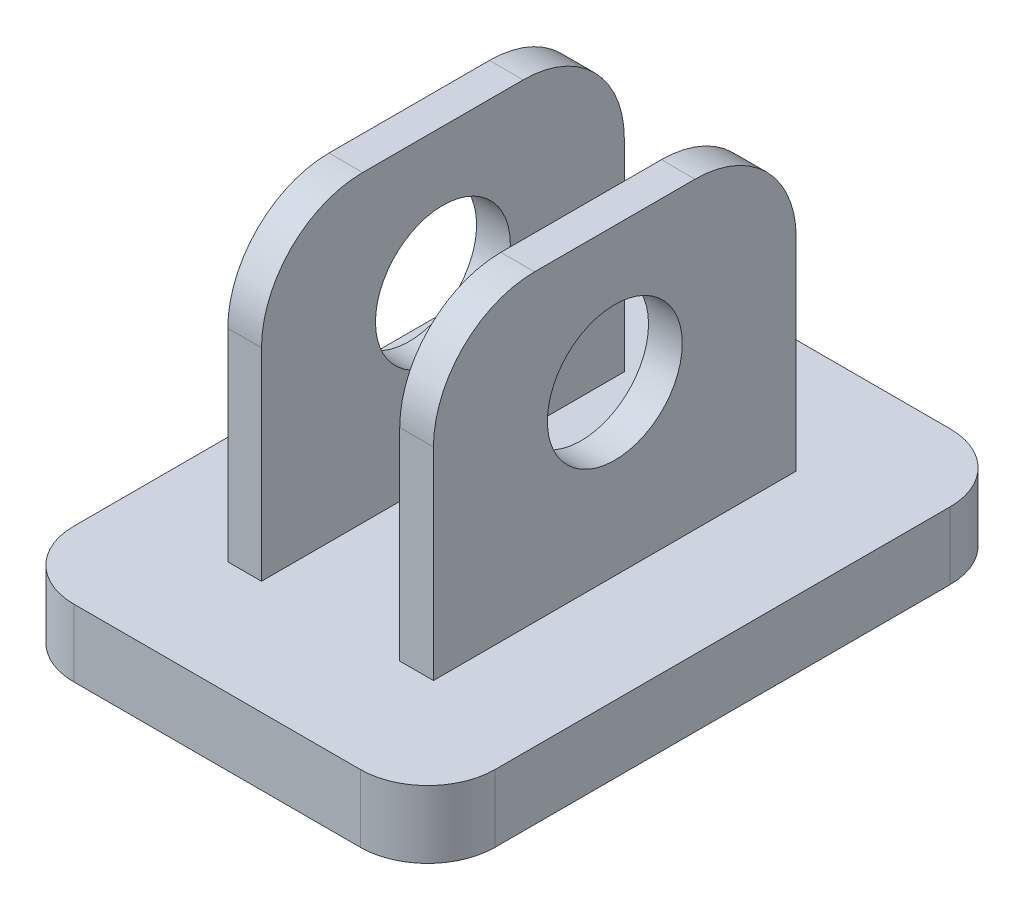
from build123d import *

# Parameters (mm, degrees)
BOSS_EXTRU_1_DEPTH = 4
SKETCH2_W          = 2
SKETCH2_H          = 21.522663516
BOSS_EXTRU_2_DEPTH = 18
FILLET1_R          = 6
SKETCH3_R          = 4
CUT_EXTRUDE1_DEPTH = 34.707714251


with BuildPart() as part:
    # Sketch1 → Boss.-Extru.1 (new body)
    with BuildSketch(Plane(origin=(0, 0, 0), x_dir=(1, 0, 0), z_dir=(0, 1, 0))):
        with BuildLine():
            Line((-8.5, -17.5), (8.5, -17.5))
            ThreePointArc((8.5, -17.5), (11.328427125, -16.328427125), (12.5, -13.5))
            Line((12.5, -13.5), (12.5, 13.5))
            ThreePointArc((12.5, 13.5), (11.328427125, 16.328427125), (8.5, 17.5))
            Line((8.5, 17.5), (-8.5, 17.5))
            ThreePointArc((-8.5, 17.5), (-11.328427125, 16.328427125), (-12.5, 13.5))
            Line((-12.5, 13.5), (-12.5, -13.5))
            ThreePointArc((-12.5, -13.5), (-11.328427125, -16.328427125), (-8.5, -17.5))
        make_face()
    extrude(amount=BOSS_EXTRU_1_DEPTH)

    # Sketch2 → Boss.-Extru.2 (add)
    with BuildSketch(Plane(origin=(0, 4, 0), x_dir=(1, 0, 0), z_dir=(0, 1, 0))):
        with Locations((-5.1, 0)):
            Rectangle(SKETCH2_W, SKETCH2_H)
        with Locations((5.1, 0)):
            Rectangle(SKETCH2_W, SKETCH2_H)
    extrude(amount=BOSS_EXTRU_2_DEPTH)

    # Fillet1
    fillet1_edges = [part.edges().sort_by_distance(p)[0] for p in [
        (5.1, 22, -10.761331758),
        (5.1, 22, 10.761331758),
        (-5.1, 22, -10.761331758),
        (-5.1, 22, 10.761331758),
    ]]
    fillet(fillet1_edges, radius=FILLET1_R)

    # Sketch3 → Cut-Extrude1 (cut, through all)
    with BuildSketch(Plane(origin=(6.1, 0, 0), x_dir=(0, 0, -1), z_dir=(1, 0, 0))):
        with Locations((0, 13.939258033)):
            Circle(SKETCH3_R)
    extrude(amount=-CUT_EXTRUDE1_DEPTH, mode=Mode.SUBTRACT)


solid = part.part
